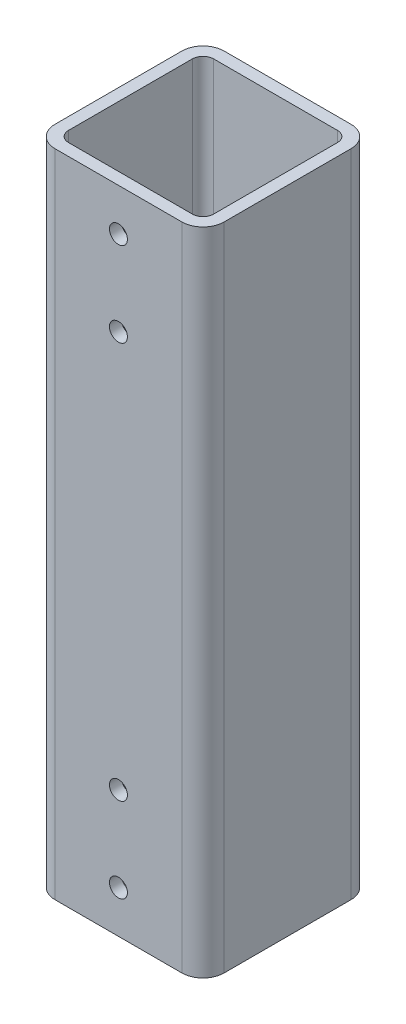
SolidWorks part; units mm, degrees
ref_plane "Front Plane" through (0, 0, 0) normal (0, 0, 1) x (1, 0, 0)
ref_plane "Top Plane" through (0, 0, 0) normal (0, 1, 0) x (1, 0, 0)
ref_plane "Right Plane" through (0, 0, 0) normal (1, 0, 0) x (0, 0, -1)
ref_plane "Plane4" through (-35, 0, 0) normal (-1, 0, 0) x (0, -1, 0)
sketch "Sketch1" plane through (-35, 0, 0) normal (-1, 0, 0) x (0, -1, 0)
  line L0 (249.1429, -40) -> (249.1429, 40)
  line L1 (249.1429, 40) -> (-58.4971, 40)
  line L2 (-58.4971, 40) -> (-58.4971, -40)
  line L3 (-58.4971, -40) -> (249.1429, -40)
  dimension "D1" = 80
  dimension "D2" = 307.64
extrude "Boss-Extrude1" add sketch "Sketch1" against normal blind 80
sketch "Sketch2" plane through (0, -249.1429, 0) normal (0, -1, 0) x (1, 0, 0)
  line L0 (-29.3, -34.3) -> (39.3, -34.3)
  line L1 (39.3, -34.3) -> (39.3, 34.3)
  line L2 (39.3, 34.3) -> (-29.3, 34.3)
  line L3 (-29.3, 34.3) -> (-29.3, -34.3)
  line L4 (-35, -40) -> (-35, 40) construction
  line L5 (45, 40) -> (-35, 40) construction
  line L6 (45, -40) -> (45, 40) construction
  line L7 (45, -40) -> (-35, -40) construction
  dimension "D1" = 5.7
  dimension "D2" = 5.7
  dimension "D3" = 5.7
  dimension "D4" = 5.7
extrude "Cut-Extrude1" cut sketch "Sketch2" against normal through all
hole_wizard "Ø8.5 (8.5) Diameter Hole2" positions "Sketch6" profile "Sketch5" hole size "Ø8.5" standard "ANSI Metric"
sketch "Sketch6" plane through (0, 0, 40) normal (0, 0, 1) x (1, 0, 0)
  line L0 (45, -249.1429) -> (45, 58.4971) construction
  line L1 (45, -249.1429) -> (-35, -249.1429) construction
  point P0 (5, -189.1429)
  point P1 (5, -229.1429)
  dimension "D1" = 40
  dimension "D2" = 40
  dimension "D3" = 40
  dimension "D4" = 60
sketch "Sketch5" plane through (5, -189.1429, 40) normal (1, 0, 0) x (0, -1, 0)
  line L0 (0, 0) -> (0, 5.7)
  line L1 (0, 5.7) -> (4.25, 5.7)
  line L2 (4.25, 5.7) -> (4.25, 0)
  line L5 (4.25, 0) -> (0, 0)
  line L11 (0, -6.35) -> (0, 107.95) construction
  dimension "通孔孔直径" = 8.5
  dimension "通孔孔深度" = 5.7
fillet "Fillet1" radius 5 4 edges at (39.3, -95.3229, 34.3) (-29.3, -95.3229, 34.3) (39.3, -95.3229, -34.3) (-29.3, -95.3229, -34.3)
fillet "Fillet2" radius 10 4 edges at (-35, -95.3229, 40) (-35, -95.3229, -40) (45, -95.3229, 40) (45, -95.3229, -40)
hole_wizard "Ø8.5 (8.5) Diameter Hole3" positions "Sketch7" profile "Sketch8" hole size "Ø8.5" standard "ANSI Metric"
sketch "Sketch7" plane through (0, 0, 40) normal (0, 0, 1) x (1, 0, 0)
  line L0 (35, 58.4971) -> (-25, 58.4971) construction
  line L2 (45, -249.1429) -> (45, 58.4971) construction
  point P0 (5, 38.4971)
  dimension "D1" = 20
  dimension "D2" = 40
sketch "Sketch8" plane through (5, 38.4971, 40) normal (1, 0, 0) x (0, -1, 0)
  line L0 (0, 0) -> (0, 12.5537)
  line L1 (0, 12.5537) -> (4.25, 10)
  line L2 (4.25, 10) -> (4.25, 0)
  line L5 (4.25, 0) -> (0, 0)
  line L10 (0, 12.5537) -> (-4.25, 10) construction
  line L11 (0, -6.35) -> (0, 107.95) construction
  dimension "孔直径" = 8.5
  dimension "孔深度" = 10
  dimension "导头角度" = 118
hole_wizard "Ø8.5 (8.5) Diameter Hole5" positions "Sketch11" profile "Sketch12" hole size "Ø8.5" standard "ANSI Metric"
sketch "Sketch11" plane through (0, 0, 40) normal (0, 0, 1) x (1, 0, 0)
  line L0 (45, 58.4971) -> (45, -249.1429) construction
  line L1 (35, 58.4971) -> (-25, 58.4971) construction
  point P0 (5, -1.5029)
  dimension "D1" = 40
  dimension "D2" = 60
sketch "Sketch12" plane through (5, -1.5029, 40) normal (1, 0, 0) x (0, -1, 0)
  line L0 (0, 0) -> (0, 12.5537)
  line L1 (0, 12.5537) -> (4.25, 10)
  line L2 (4.25, 10) -> (4.25, 0)
  line L5 (4.25, 0) -> (0, 0)
  line L10 (0, 12.5537) -> (-4.25, 10) construction
  line L11 (0, -6.35) -> (0, 107.95) construction
  dimension "孔直径" = 8.5
  dimension "孔深度" = 10
  dimension "导头角度" = 118
